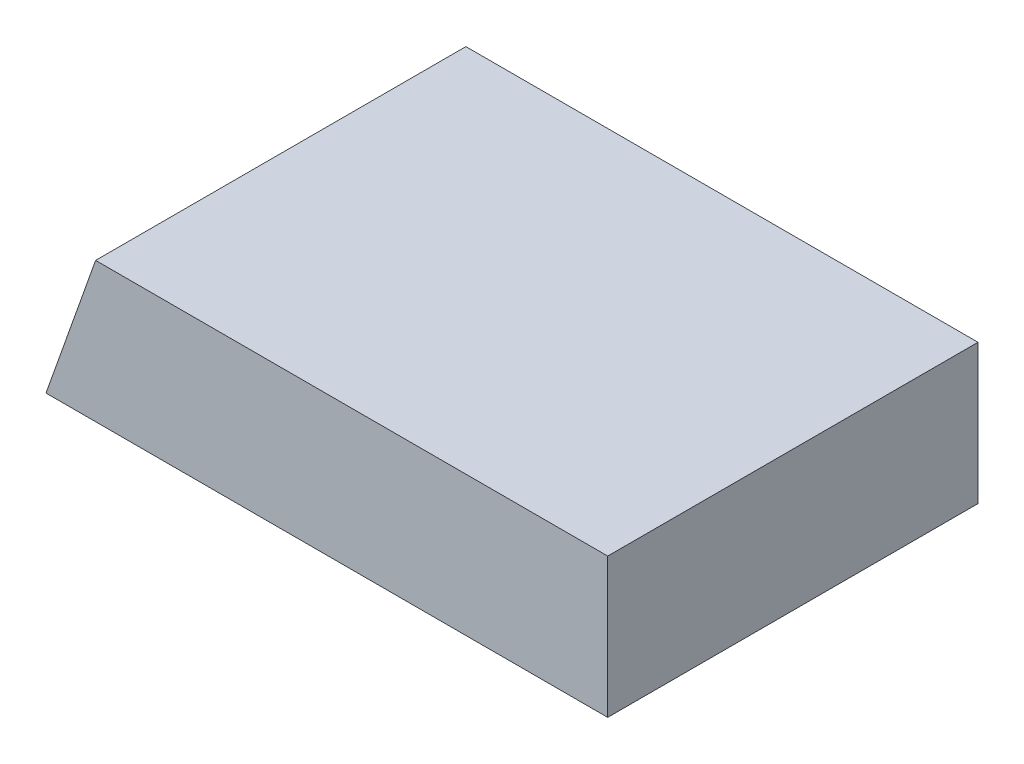
from build123d import *

# Parameters (mm, degrees)
EXTRUDE_1_DEPTH = 26.5


with BuildPart() as part:
    # 草图1 → 凸台-拉伸1 (new, symmetric)
    with BuildSketch(Plane.XY):
        Polygon((0, 0), (0, 20), (-73.3, 20), (-80.4, 0), align=None)
    extrude(amount=EXTRUDE_1_DEPTH, both=True)


solid = part.part
